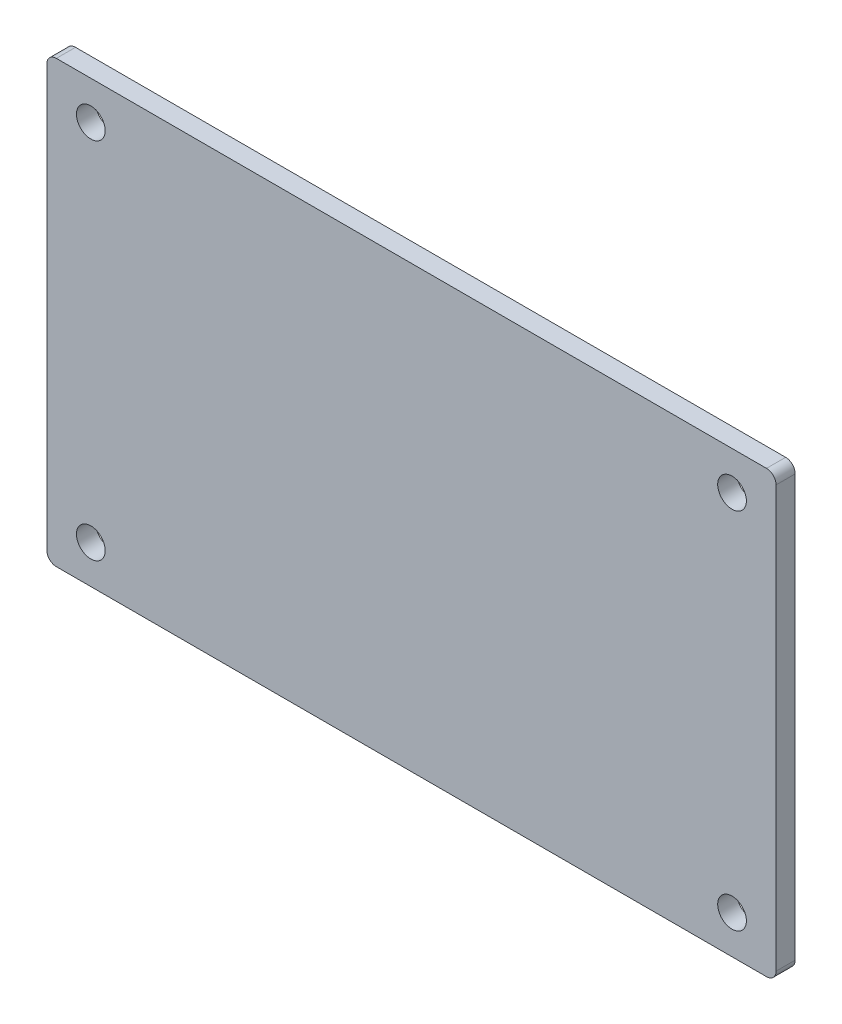
from build123d import *

# Parameters (mm, degrees)
SKETCH1_W           = 381
SKETCH1_H           = 230
BOSS_EXTRUDE1_DEPTH = 5
F_15_HOLE1_D        = 15
FILLET2_R           = 5


with BuildPart() as part:
    # Sketch1 → Boss-Extrude1 (new, symmetric)
    with BuildSketch(Plane.XY):
        Rectangle(SKETCH1_W, SKETCH1_H)
    extrude(amount=BOSS_EXTRUDE1_DEPTH, both=True)

    # Ø15 Hole1 (through all)
    with Locations(Plane.XY.offset(5)):
        with Locations((-167.5, 95), (167.5, 95), (167.5, -95), (-167.5, -95)):
            Hole(F_15_HOLE1_D / 2)

    # Fillet2
    fillet2_edges = [part.edges().sort_by_distance(p)[0] for p in [
        (-190.5, 115, 0),
        (190.5, 115, 0),
        (190.5, -115, 0),
        (-190.5, -115, 0),
    ]]
    fillet(fillet2_edges, radius=FILLET2_R)


solid = part.part
